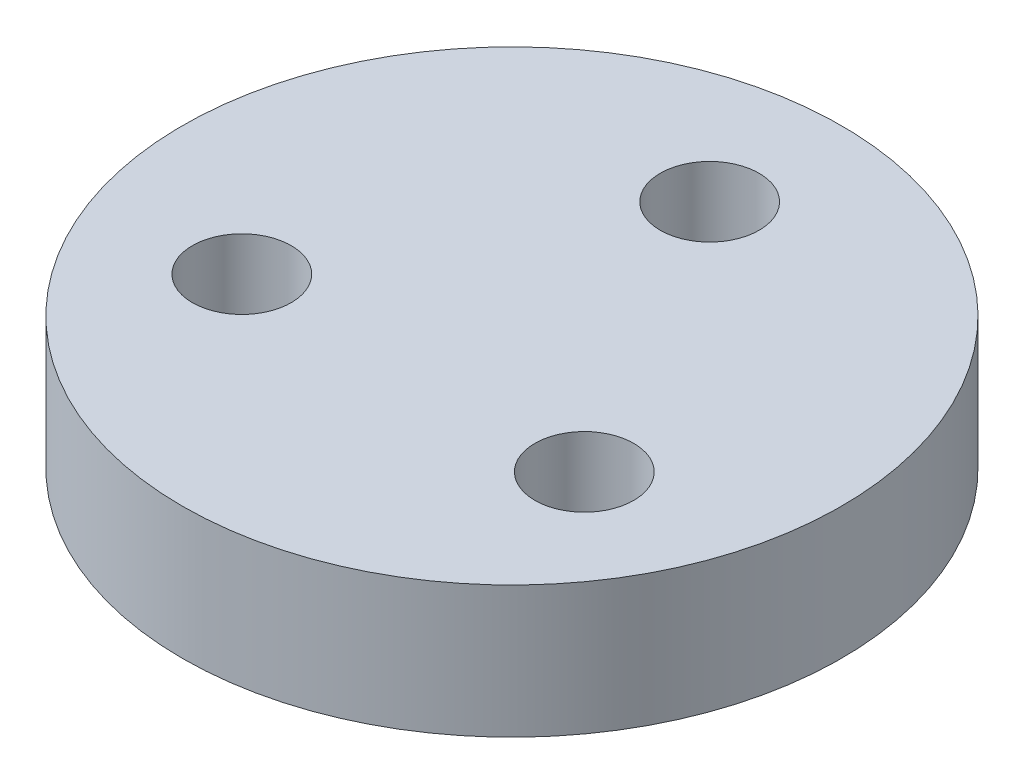
SolidWorks part; units mm, degrees
ref_plane "Front Plane" through (0, 0, 0) normal (0, 0, 1) x (1, 0, 0)
ref_plane "Top Plane" through (0, 0, 0) normal (0, 1, 0) x (1, 0, 0)
ref_plane "Right Plane" through (0, 0, 0) normal (1, 0, 0) x (0, 0, -1)
sketch "Sketch1" plane through (0, 0, 0) normal (0, 1, 0) x (1, 0, 0)
  circle A0 centre (0, 0) radius 50
  dimension "D1" = 100
extrude "Boss-Extrude1" add sketch "Sketch1" along normal blind 20
sketch "Sketch2" plane through (0, 20, 0) normal (0, 1, 0) x (1, 0, 0)
  circle A0 centre (0, 30) radius 7.5
  circle A1 centre (25.9808, -15) radius 7.5
  circle A2 centre (-25.9808, -15) radius 7.5
  point P10 (0, 0)
  dimension "D1" = 15
  dimension "D2" = 30
  dimension "D3" = 3
extrude "Cut-Extrude1" cut sketch "Sketch2" against normal blind 15
sketch "Sketch3" plane through (0, 0, 0) normal (0, -1, 0) x (1, 0, 0)
  circle A0 centre (25.9808, 15) radius 4 construction
  circle A1 centre (-25.9808, 15) radius 4 construction
  circle A2 centre (0, -30) radius 4 construction
  circle A3 centre (25.9808, 19) radius 1
  circle A4 centre (29.9808, 15) radius 1
  circle A5 centre (21.9808, 15) radius 1
  circle A6 centre (25.9808, 11) radius 1
  circle A7 centre (-25.9808, 19) radius 1
  circle A8 centre (-29.9808, 15) radius 1
  circle A9 centre (-25.9808, 11) radius 1
  circle A10 centre (-21.9808, 15) radius 1
  circle A11 centre (0, -26) radius 1
  circle A12 centre (-4, -30) radius 1
  circle A13 centre (0, -34) radius 1
  circle A14 centre (4, -30) radius 1
  dimension "D1" = 8
  dimension "D2" = 8
  dimension "D3" = 8
  dimension "D4" = 2
  dimension "D5" = 2
  dimension "D6" = 2
  dimension "D7" = 2
  dimension "D8" = 2
  dimension "D9" = 2
  dimension "D10" = 2
  dimension "D11" = 2
  dimension "D12" = 2
  dimension "D13" = 2
  dimension "D14" = 2
  dimension "D15" = 2
extrude "Cut-Extrude2" cut sketch "Sketch3" against normal through all
sketch "Sketch4" plane through (0, 0, 0) normal (0, -1, 0) x (1, 0, 0)
  circle A0 centre (-25.9808, 19) radius 1.8
  circle A1 centre (-29.9808, 15) radius 1.8
  circle A2 centre (-25.9808, 11) radius 1.8
  circle A3 centre (-21.9808, 15) radius 1.8
  circle A4 centre (25.9808, 19) radius 1.8
  circle A5 centre (21.9808, 15) radius 1.8
  circle A6 centre (25.9808, 11) radius 1.8
  circle A7 centre (29.9808, 15) radius 1.8
  circle A8 centre (0, -26) radius 1.8
  circle A9 centre (-4, -30) radius 1.8
  circle A10 centre (0, -34) radius 1.8
  circle A11 centre (4, -30) radius 1.8
  dimension "D1" = 3.6
extrude "Cut-Extrude3" cut sketch "Sketch4" against normal blind 4
